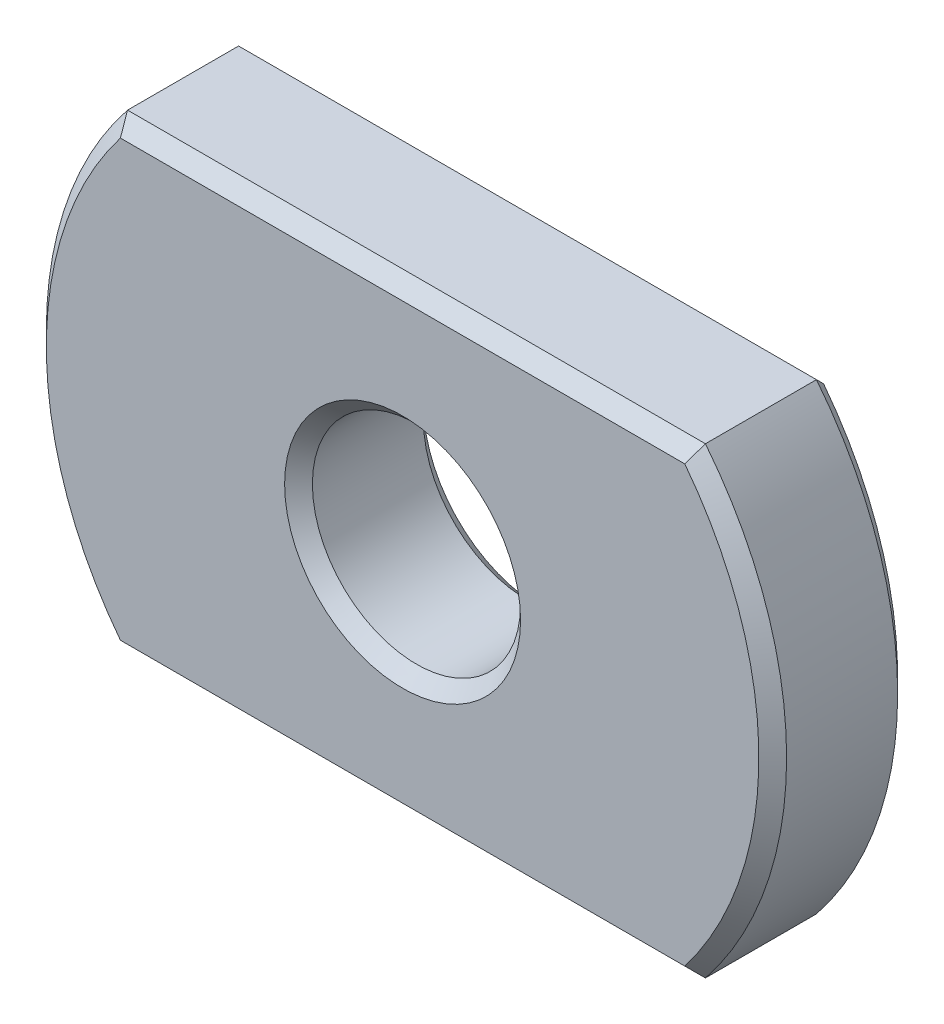
SolidWorks part; units mm, degrees
ref_plane "Front Plane" through (0, 0, 0) normal (0, 0, 1) x (1, 0, 0)
ref_plane "Top Plane" through (0, 0, 0) normal (0, 1, 0) x (1, 0, 0)
ref_plane "Right Plane" through (0, 0, 0) normal (1, 0, 0) x (0, 0, -1)
sketch "Sketch1" plane through (0, 0, 0) normal (0, 0, 1) x (1, 0, 0)
  circle A0 centre (0, 0) radius 2.25
  circle A1 centre (0, 0) radius 8
  dimension "D1" = 16
  dimension "D2" = 4.5
extrude "Boss-Extrude1" add sketch "Sketch1" along normal mid plane 3
sketch "Sketch2" plane through (0, 0, 1.5) normal (0, 0, 1) x (1, 0, 0)
  line L1 (-10, 5) -> (10, 5)
  line L2 (-10, 5) -> (-10, -5)
  line L3 (-10, -5) -> (10, -5)
  line L4 (10, 5) -> (10, -5)
  line L5 (-10, 5) -> (10, -5) construction
  line L6 (-10, -5) -> (10, 5) construction
  point P0 (0, 0)
  dimension "D1" = 10
  dimension "D2" = 20
extrude "Cut-Extrude1" cut sketch "Sketch2" against normal through all flip side to cut
chamfer "Chamfer1" distance 0.3 angle 45 10 edges at (2.25, 0, -1.5) (2.25, 0, 1.5) (-8, 0, -1.5) (8, 0, -1.5) (-8, 0, 1.5) (8, 0, 1.5) (0, 5, -1.5) (0, -5, -1.5) (0, 5, 1.5) (0, -5, 1.5)
